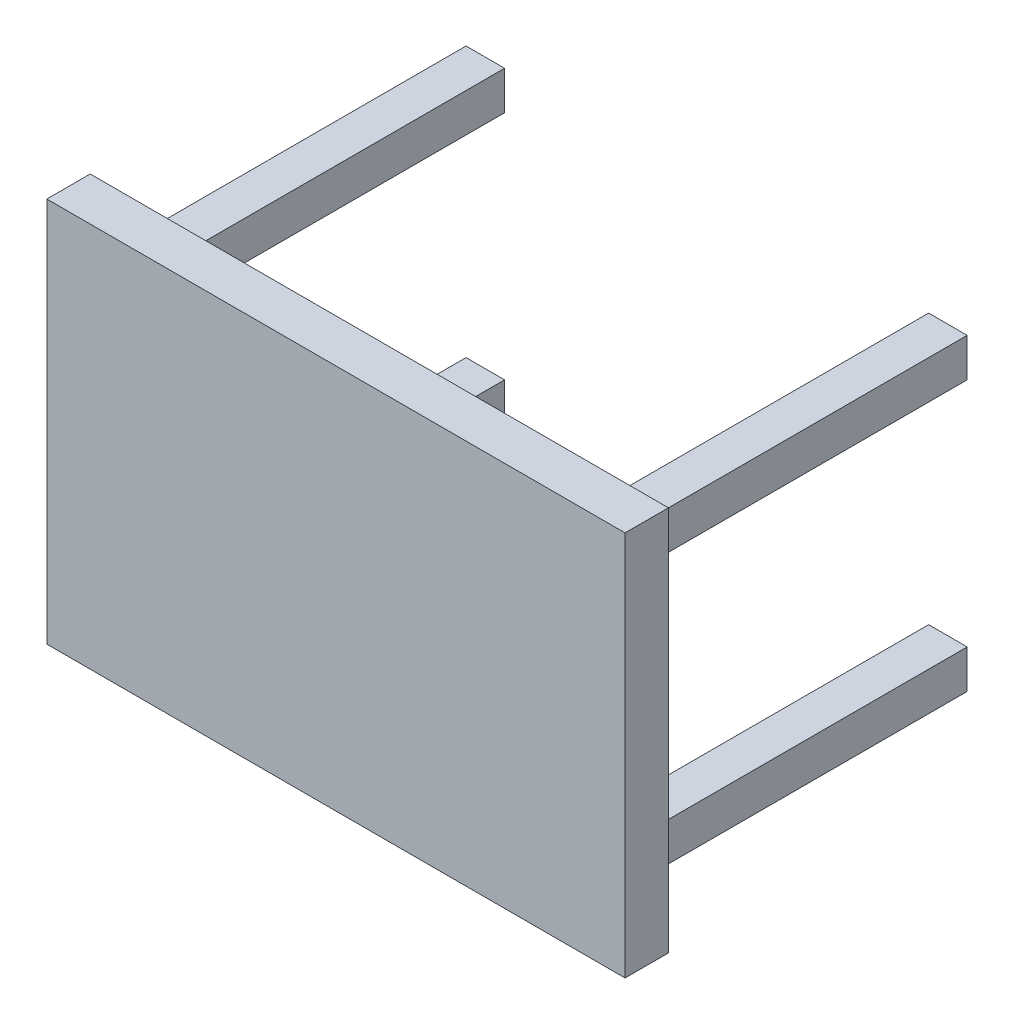
SolidWorks part; units mm, degrees
material "灰铸铁 HT250 (GB)"
ref_plane "Front Plane" through (0, 0, 0) normal (0, 0, 1) x (1, 0, 0)
ref_plane "Top Plane" through (0, 0, 0) normal (0, 1, 0) x (1, 0, 0)
ref_plane "Right Plane" through (0, 0, 0) normal (1, 0, 0) x (0, 0, -1)
sketch "Sketch1" plane through (0, 0, 0) normal (0, 0, 1) x (1, 0, 0)
  line L1 (600, -400) -> (-600, -400)
  line L2 (600, -400) -> (600, 400)
  line L3 (600, 400) -> (-600, 400)
  line L4 (-600, -400) -> (-600, 400)
  line L5 (600, -400) -> (-600, 400) construction
  line L6 (600, 400) -> (-600, -400) construction
  point P0 (0, 0)
  dimension "D1" = 1200
  dimension "D2" = 800
extrude "Boss-Extrude1" add sketch "Sketch1" against normal blind 90
sketch "Sketch2" plane through (0, 0, -90) normal (0, 0, -1) x (-1, 0, 0)
  line L0 (600, 400) -> (600, -400) construction
  line L1 (520, -320) -> (440, -320)
  line L2 (520, -320) -> (520, -240)
  line L3 (520, -240) -> (440, -240)
  line L4 (440, -320) -> (440, -240)
  line L5 (600, -400) -> (-600, -400) construction
  dimension "D1" = 80
  dimension "D2" = 80
  dimension "D3" = 80
extrude "Boss-Extrude2" add sketch "Sketch2" along normal blind 700
mirror "Mirror1" about plane through (0, 0, 0) normal (0, 1, 0) of "Boss-Extrude2"
mirror "Mirror2" about plane through (0, 0, 0) normal (1, 0, 0) of "Mirror1", "Boss-Extrude2"
